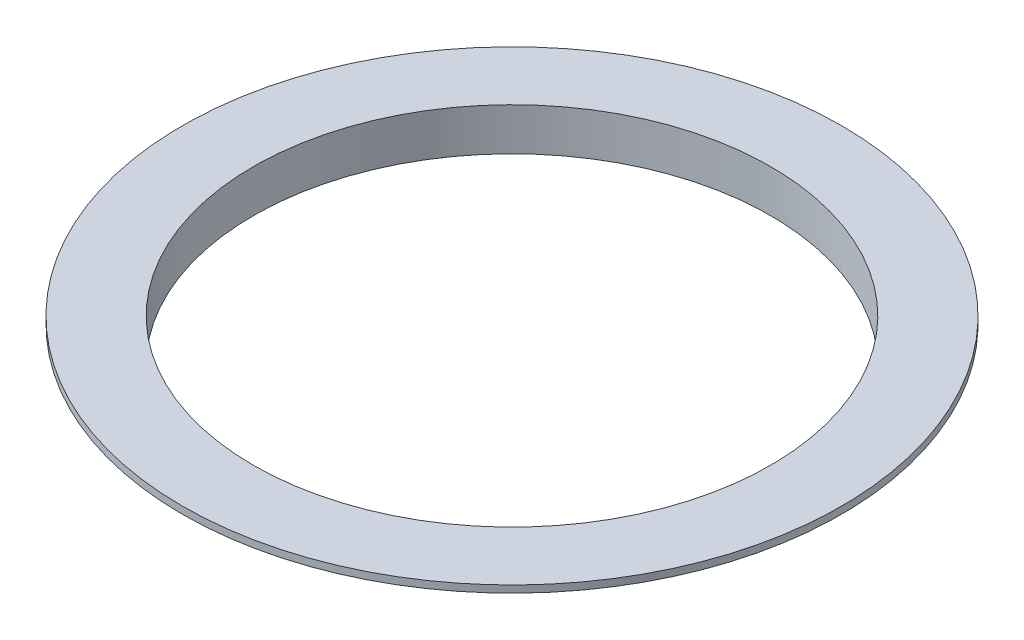
SolidWorks part; units mm, degrees
ref_plane "Front Plane" through (0, 0, 0) normal (0, 0, 1) x (1, 0, 0)
ref_plane "Top Plane" through (0, 0, 0) normal (0, 1, 0) x (1, 0, 0)
ref_plane "Right Plane" through (0, 0, 0) normal (1, 0, 0) x (0, 0, -1)
sketch "Sketch1" plane through (0, 0, 0) normal (0, 1, 0) x (1, 0, 0)
  circle A0 centre (0, 0) radius 75
  circle A1 centre (0, 0) radius 73
  dimension "D1" = 150
  dimension "D2" = 2
extrude "Boss-Extrude1" add sketch "Sketch1" along normal blind 10
sketch "Sketch3" plane through (0, 10, 0) normal (0, 1, 0) x (1, 0, 0)
  circle A0 centre (0, 0) radius 73 construction
  circle A1 centre (0, 0) radius 73
  circle A2 centre (0, 0) radius 93
  dimension "D1" = 20
extrude "Boss-Extrude2" add sketch "Sketch3" along normal blind 2
